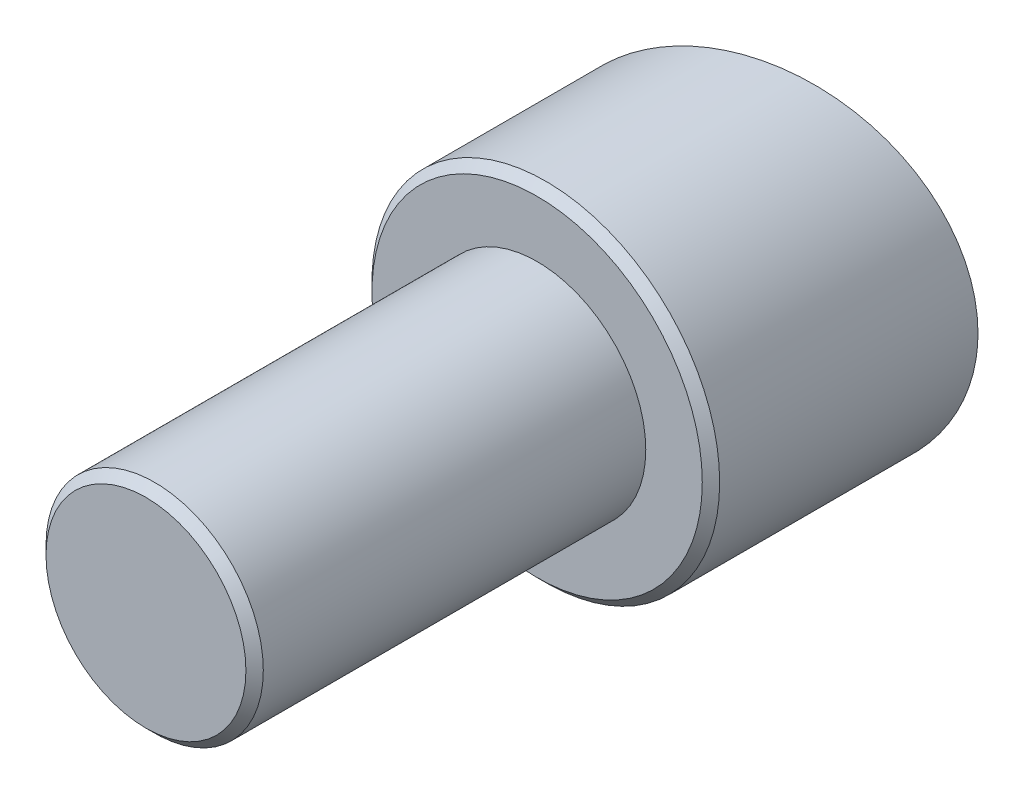
from build123d import *

# Parameters (mm, degrees)
SKETCH_1_R          = 20
EXTRUDE_1_DEPTH     = 30.72
SKETCH_2_R          = 12.5
EXTRUDE_2_DEPTH     = 45
CUT_EXTRUDE_1_DEPTH = 25
CHAMFER_1_SIZE      = 1


with BuildPart() as part:
    # 草图1 → 凸台-拉伸1 (new body)
    with BuildSketch(Plane.XY):
        Circle(SKETCH_1_R)
    extrude(amount=EXTRUDE_1_DEPTH)

    # 草图2 → 凸台-拉伸2 (add)
    with BuildSketch(Plane.XY.offset(30.72)):
        with Locations(Location((0, 0, 0), (0, 0, 180))):
            Circle(SKETCH_2_R)
    extrude(amount=EXTRUDE_2_DEPTH)

    # 草图3 → 切除-拉伸1 (cut, symmetric)
    with BuildSketch(Plane(origin=(0, 0, 0), x_dir=(1, 0, 0), z_dir=(0, 1, 0))):
        Polygon((-20, 0), (20, 0), (-20, -10.72), align=None)
    extrude(amount=CUT_EXTRUDE_1_DEPTH, both=True, mode=Mode.SUBTRACT)

    # 倒角1
    chamfer_1_edges = [part.edges().sort_by_distance(p)[0] for p in [
        (-20, 0, 30.72),
        (12.5, 0, 75.72),
    ]]
    chamfer(chamfer_1_edges, length=CHAMFER_1_SIZE)


solid = part.part
